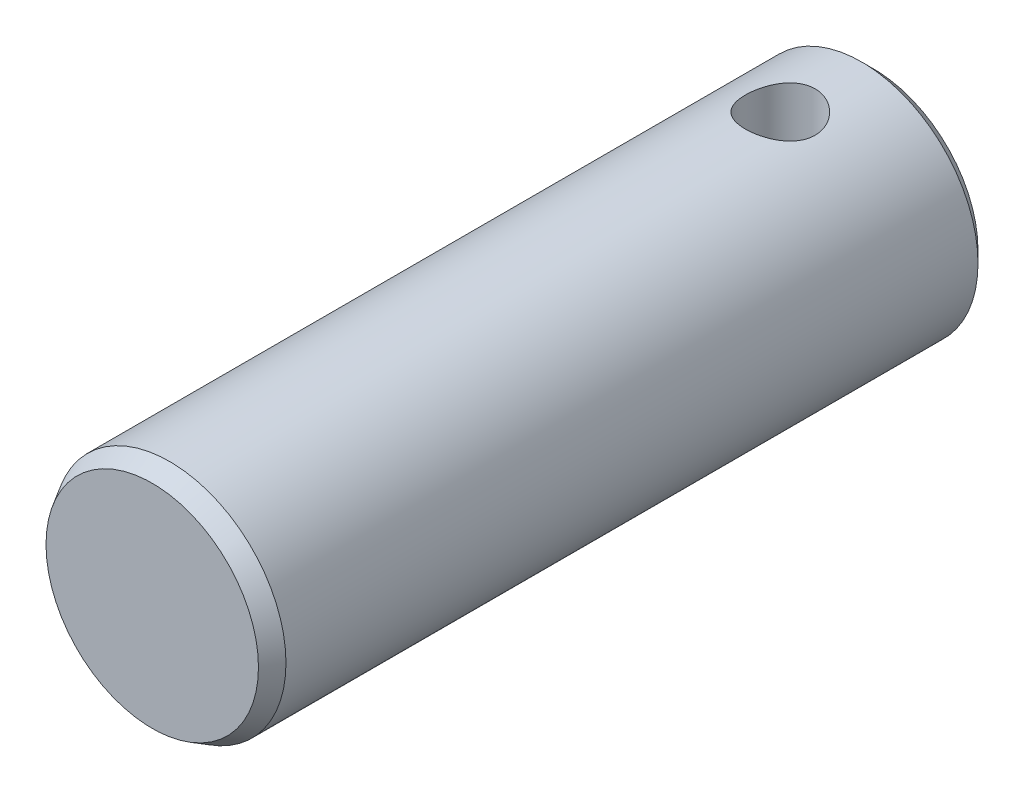
SolidWorks part; units mm, degrees
material "普通碳钢"
ref_plane "前视" through (0, 0, 0) normal (0, 0, 1) x (1, 0, 0)
ref_plane "上视" through (0, 0, 0) normal (0, 1, 0) x (1, 0, 0)
ref_plane "右视" through (0, 0, 0) normal (1, 0, 0) x (0, 0, -1)
sketch "草图1" plane through (0, 0, 0) normal (0, 0, 1) x (1, 0, 0)
  line L0 (-39.3257, 0) -> (45.1983, 0) construction
  line L1 (0, 26.1647) -> (0, -26.8988) construction
  circle A0 centre (0, 0) radius 20
  dimension "D1" = 40
extrude "凸台-拉伸1" add sketch "草图1" along normal blind 124
chamfer "倒角1" distance 3 angle 30 1 edges at (20, 0, 124)
chamfer "倒角3" distance 2 angle 45 1 edges at (20, 0, 0)
sketch "草图3" plane through (0, 0, 0) normal (0, 1, 0) x (1, 0, 0)
  line L0 (0, -121) -> (0, -2) construction
  line L1 (18, 0) -> (-18, 0) construction
  circle A0 centre (0, -16) radius 6
  dimension "D1" = 12
  dimension "D2" = 16
extrude "切除-拉伸2" cut sketch "草图3" against normal through all both and the other way through all
